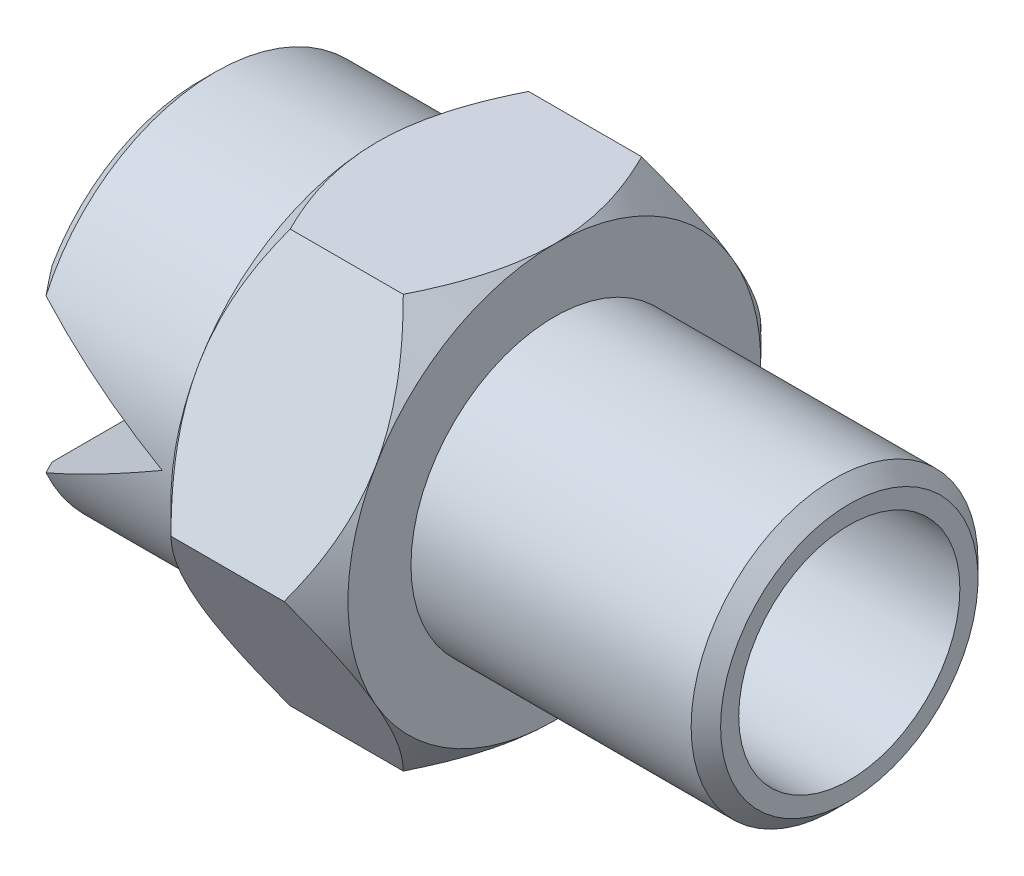
from build123d import *

# Parameters (mm, degrees)
SKETCH2_R               = 4.864
BOSS_EXTRUDE1_DEPTH     = 6
CUT_EXTRUDE1_DEPTH      = 25.460853079
CUT_EXTRUDE1_DEPTH_BACK = 25.460853079
SKETCH5_R               = 2.5
CUT_EXTRUDE2_DEPTH      = 20.244046698


with BuildPart() as part:
    # Sketch1 → Revolve1 (revolve)
    with BuildSketch(Plane.XY, mode=Mode.PRIVATE) as revolve1_sk:
        Polygon((0, 0), (0, 5.8), (0.5, 6.3), (6, 6.3), (6, 7), (12, 7), (12, 4.864), (21.5, 4.864), (22, 4.364), (22, 3.75), (6, 3.75), (6, 0), align=None)
    revolve(revolve1_sk.sketch.rotate(Axis((0, 0, 0), (1, 0, 0)), 90), axis=Axis((0, 0, 0), (1, 0, 0)))

    # Sketch2 → Boss-Extrude1 (add)
    with BuildSketch(Plane(origin=(12, 0, 0), x_dir=(0, 0, -1), z_dir=(1, 0, 0))):
        Polygon((8.082903769, 0), (4.041451884, 7), (-4.041451884, 7), (-8.082903769, 0), (-4.041451884, -7), (4.041451884, -7), align=None)
        with Locations(Location((0, 0, 0), (0, 0, 180))):
            Circle(SKETCH2_R, mode=Mode.SUBTRACT)
    extrude(amount=-BOSS_EXTRUDE1_DEPTH)

    # Sketch3 → Cut-Revolve1 (revolve, cut)
    with BuildSketch(Plane(origin=(0, 0, 0), x_dir=(1, 0, 0), z_dir=(0, 1, 0))):
        Polygon((10.917096231, 8.082903769), (12, 7), (12, 8.082903769), align=None)
        Polygon((6, 7), (7.082903769, 8.082903769), (6, 8.082903769), align=None)
    revolve(axis=Axis((0, 0, 0), (-1, 0, 0)), mode=Mode.SUBTRACT)

    # Sketch4 → Cut-Extrude1 (cut, two sides: drawn at the far end of the back side and taken through both)
    with BuildSketch(Plane.XY.offset(-CUT_EXTRUDE1_DEPTH_BACK)):
        Polygon((0, 2.886751346), (5, 0), (0, -2.886751346), align=None)
    extrude(amount=CUT_EXTRUDE1_DEPTH + CUT_EXTRUDE1_DEPTH_BACK, mode=Mode.SUBTRACT)

    # Sketch5 → Cut-Extrude2 (cut, through all)
    with BuildSketch(Plane(origin=(6, 0, 0), x_dir=(0, 0, -1), z_dir=(1, 0, 0))):
        Circle(SKETCH5_R)
    extrude(amount=-CUT_EXTRUDE2_DEPTH, mode=Mode.SUBTRACT)


solid = part.part
